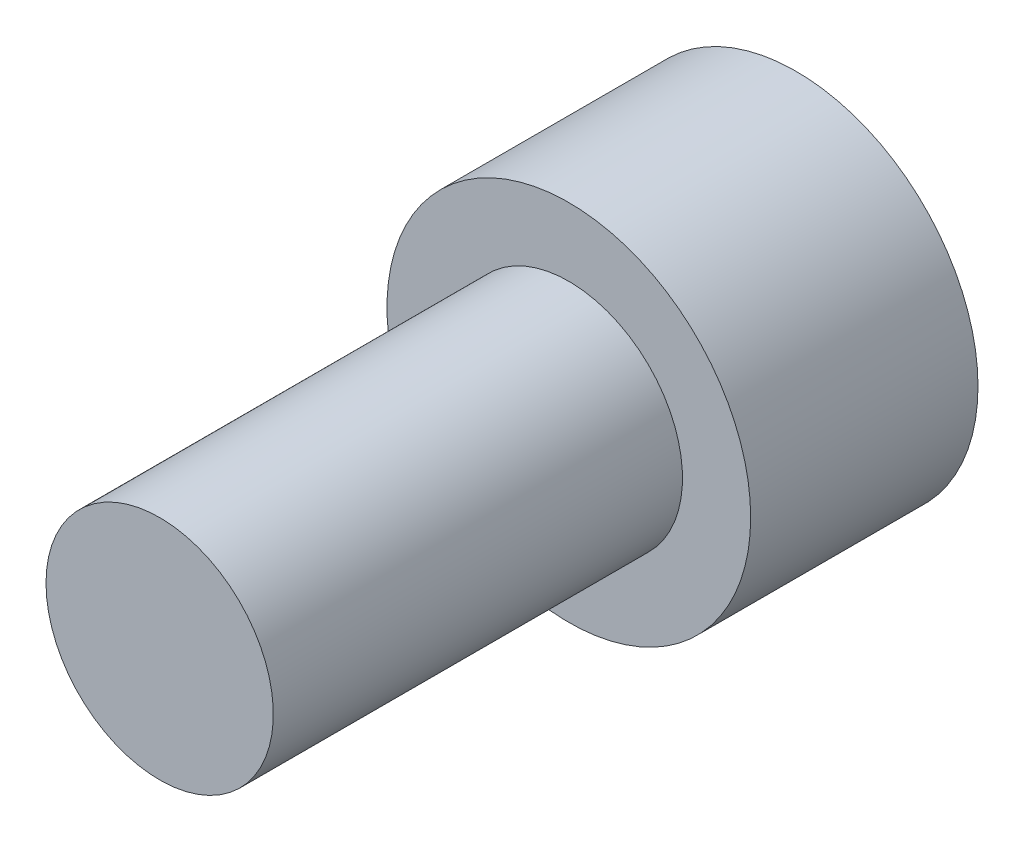
SolidWorks part; units mm, degrees
ref_plane "前视基准面" through (0, 0, 0) normal (0, 0, 1) x (1, 0, 0)
ref_plane "上视基准面" through (0, 0, 0) normal (0, 1, 0) x (1, 0, 0)
ref_plane "右视基准面" through (0, 0, 0) normal (1, 0, 0) x (0, 0, -1)
sketch "草图1" plane through (0, 0, 0) normal (0, 0, 1) x (1, 0, 0)
  circle A0 centre (0, 0) radius 20
  dimension "D1" = 40
extrude "凸台-拉伸1" add sketch "草图1" along normal blind 25
sketch "草图2" plane through (0, 0, 25) normal (0, 0, 1) x (1, 0, 0)
  circle A0 centre (0, 0) radius 12.5
  dimension "D1" = 25
extrude "凸台-拉伸2" add sketch "草图2" along normal blind 45
